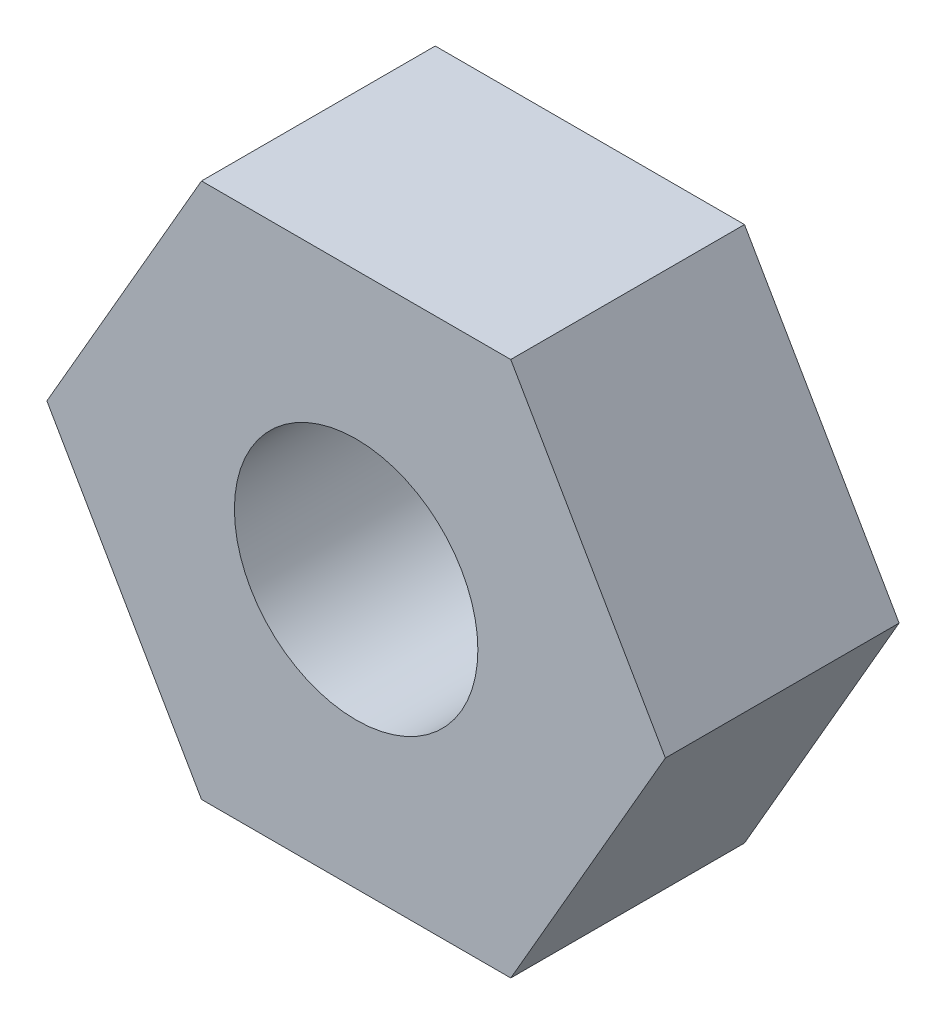
from build123d import *

# Parameters (mm, degrees)
SKETCH_1_R      = 1.25
EXTRUDE_1_DEPTH = 1.2


with BuildPart() as part:
    # 草图1 → 凸台-拉伸1 (new, symmetric)
    with BuildSketch(Plane.XY):
        Polygon((3.175426481, 0), (1.58771324, 2.75), (-1.58771324, 2.75), (-3.175426481, 0), (-1.58771324, -2.75), (1.58771324, -2.75), align=None)
        Circle(SKETCH_1_R, mode=Mode.SUBTRACT)
    extrude(amount=EXTRUDE_1_DEPTH, both=True)


solid = part.part
